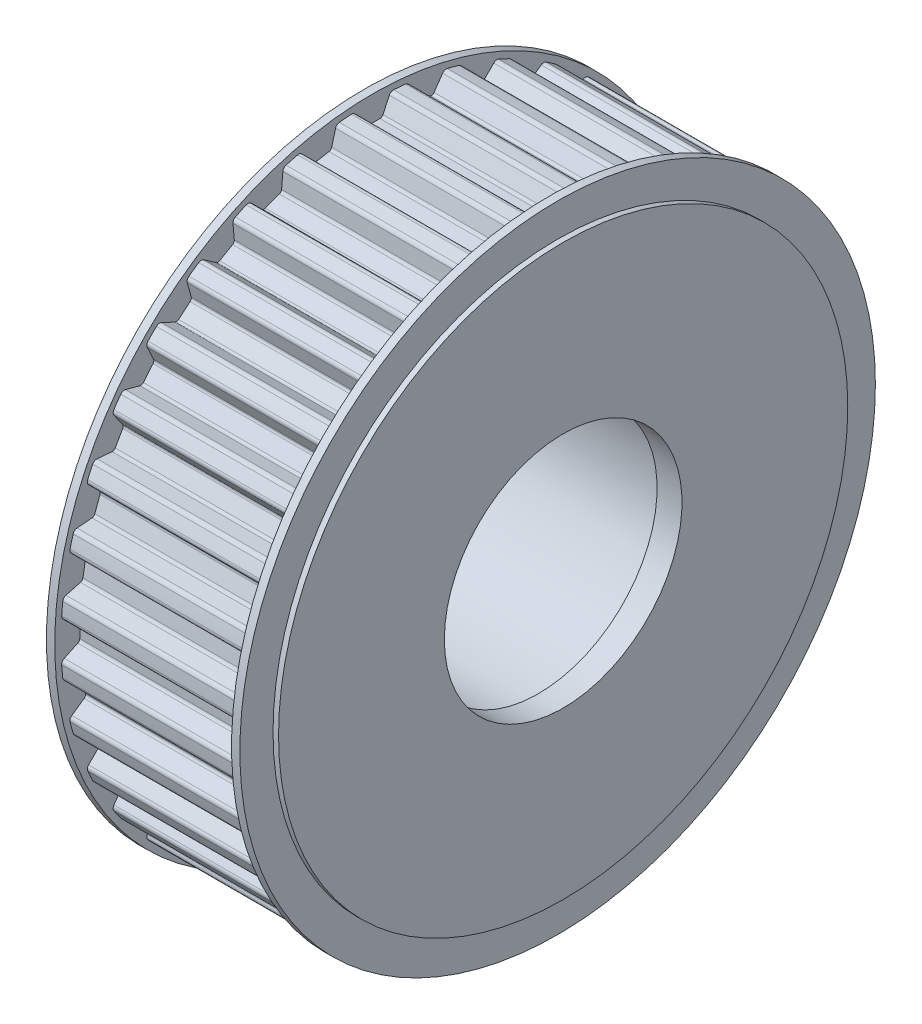
SolidWorks part; units mm, degrees
material "6061 合金"
ref_plane "前视" through (0, 0, 0) normal (0, 0, 1) x (1, 0, 0)
ref_plane "上视" through (0, 0, 0) normal (0, 1, 0) x (1, 0, 0)
ref_plane "右视" through (0, 0, 0) normal (1, 0, 0) x (0, 0, -1)
sketch "草图1" plane through (0, 0, 0) normal (1, 0, 0) x (0, 0, -1)
  line L0 (0, 56.37) -> (0, 56.751) construction
  circle A1 centre (0, 0) radius 56.37
  circle A2 centre (0, 0) radius 56.751 construction
  dimension "D2" = 112.74
  dimension "D3" = 0.381
extrude "拉伸1" add sketch "草图1" along normal mid plane 32
sketch "草图2" plane through (16, 0, 0) normal (1, 0, 0) x (0, 0, -1)
  line L0 (0, 0) -> (0, 61.5267) construction
  line L1 (-3.285, 56.2742) -> (-1.7442, 52.97)
  line L2 (-1.7442, 52.97) -> (1.7442, 52.97)
  line L3 (1.7442, 52.97) -> (3.285, 56.2742)
  circle A0 centre (0, 0) radius 56.37 construction
  arc A1 (3.285, 56.2742) -> (-3.285, 56.2742) centre (0, 0) ccw
  dimension "D2" = 3.4
  dimension "D3" = 25
  dimension "D1" = 6.57
extrude "拉伸2" cut sketch "草图2" against normal up to surface (32 mm away) up to face at (-16, 0, -56.37)
fillet "圆角1" radius 0.6 2 edges at (0, 52.97, -1.7442) (0, 52.97, 1.7442)
fillet "圆角2" radius 0.8 2 edges at (0, 56.2742, -3.285) (0, 56.2742, 3.285)
pattern_circular "阵列(圆周)1" count 36 over 360 about axis through (0, 0, 0) along (1, 0, 0) of "拉伸2", "圆角1", "圆角2"
sketch "草图6" plane through (16, 0, 0) normal (1, 0, 0) x (0, 0, -1)
  circle A0 centre (0, 0) radius 57.5
  dimension "D1" = 115
extrude "凸台-拉伸2" add sketch "草图6" along normal blind 1.5
sketch "草图7" plane through (17.5, 0, 0) normal (1, 0, 0) x (0, 0, -1)
  circle A0 centre (0, 0) radius 51.5
  dimension "D1" = 103
extrude "凸台-拉伸3" add sketch "草图7" along normal blind 1
mirror "镜向2" about plane through (0, 0, 0) normal (1, 0, 0) of "凸台-拉伸3", "凸台-拉伸2"
sketch "草图8" plane through (-18.5, 0, 0) normal (-1, 0, 0) x (0, 0, 1)
  circle A0 centre (0, 0) radius 21.5
  dimension "D1" = 43
extrude "切除-拉伸1" cut sketch "草图8" against normal through all
sketch "草图9" plane through (-18.5, 0, 0) normal (-1, 0, 0) x (0, 0, 1)
  circle A0 centre (0, 0) radius 23.5
  dimension "D1" = 47
extrude "切除-拉伸2" cut sketch "草图9" against normal blind 32.5
sketch "草图10" plane through (0, 0, 0) normal (0, 1, 0) x (1, 0, 0)
  line L0 (14, 23.5) -> (-18.5, 23.5) construction
  line L1 (-15.8, 23.5) -> (-14, 23.5)
  line L2 (-15.8, 23.5) -> (-15.8, 24.75)
  line L3 (-15.8, 24.75) -> (-14, 24.75)
  line L4 (-14, 23.5) -> (-14, 24.75)
  line L5 (14, 23.5) -> (14, -23.5) construction
  line L6 (0, 0) -> (-33.3455, 0) construction
  dimension "D1" = 1.8
  dimension "D2" = 28
  dimension "D3" = 24.75
revolve "切除-旋转1" cut sketch "草图10" angle 360 about L6
